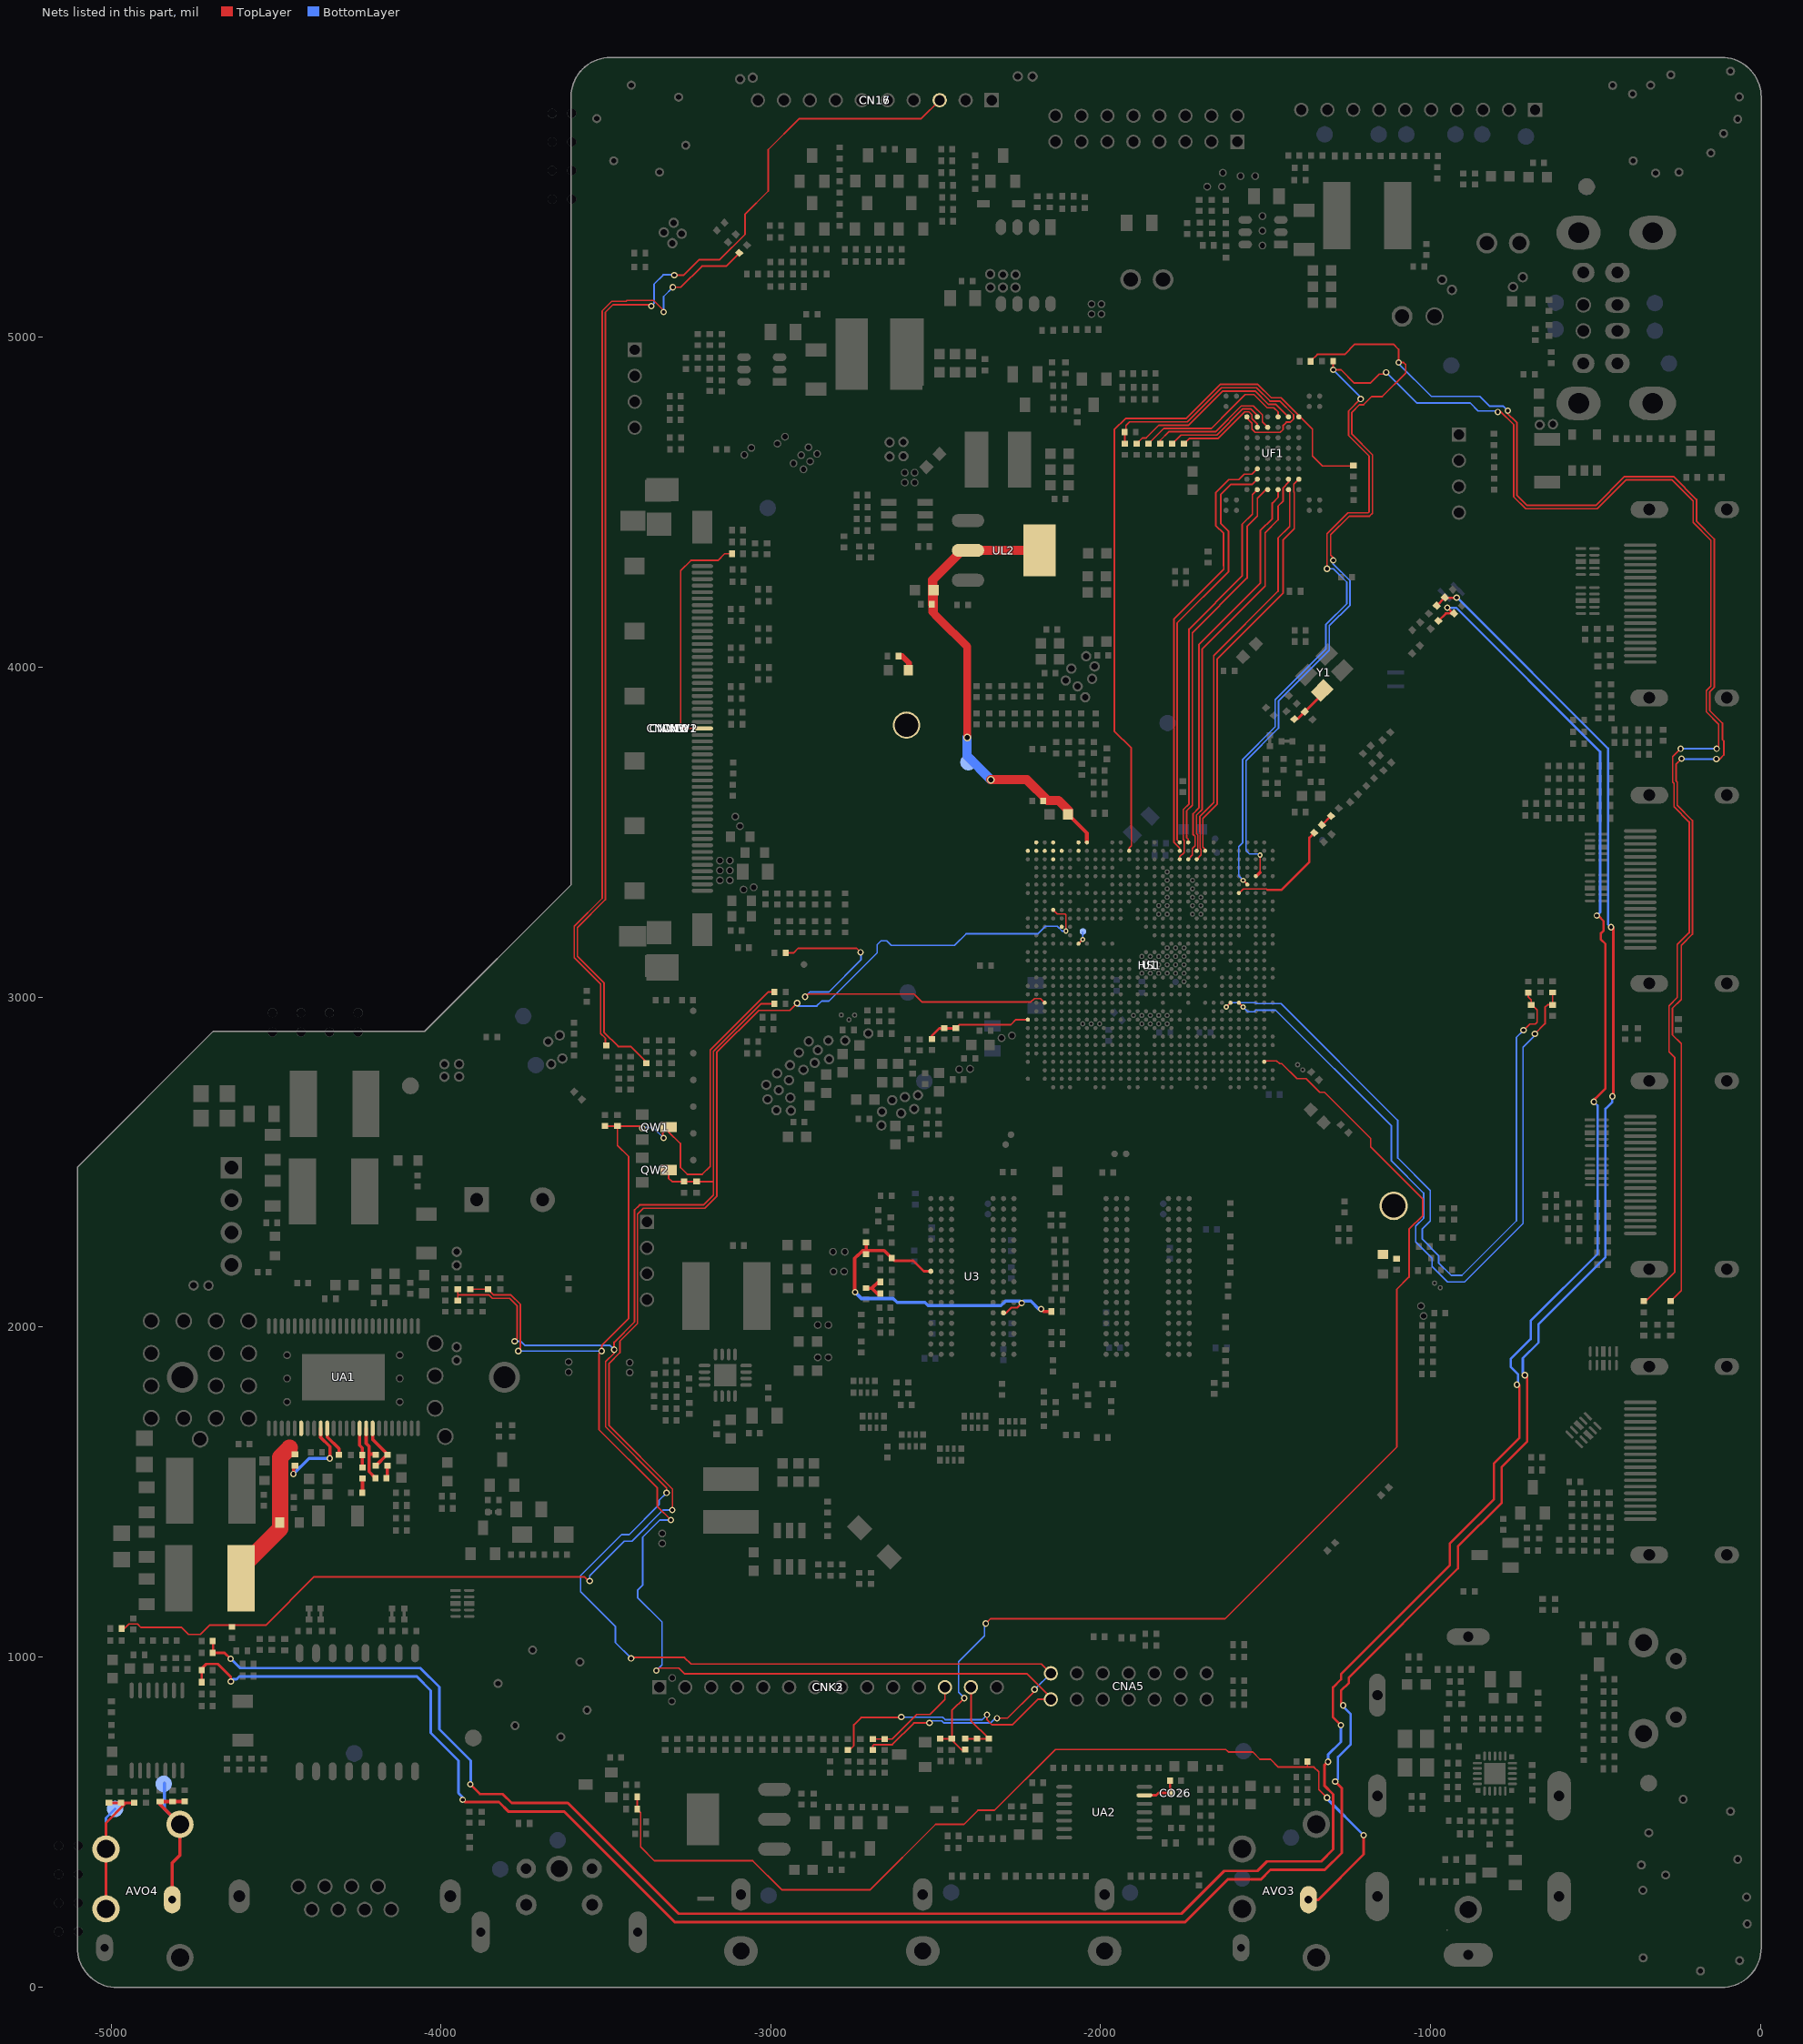
[diagram p0: the nets of this part, all layers, seen from the top]
# Altium PCB MISC86290.PcbDoc (part 24 of 31)
Units mil, origin at the board's own origin, x right, y up, seen from the top; angles counter-clockwise.
Board outline 5104.71 x 5851.49 mil, 2 copper layers (TopLayer, BottomLayer), stack 61.855 mil thick; 1026 components, 667 nets, 4280 pads, 2294 vias.

## Via types
v1: diameter 19.68, hole 11.81, TopLayer to BottomLayer, tented both sides, 1189 vias
v2: diameter 19.68/19.68 (per signal layer), hole 11.81, TopLayer to BottomLayer, tented both sides, 366 vias
v3: diameter 15.75, hole 7.87, TopLayer to BottomLayer, tented both sides, 348 vias
v4: diameter 23.62, hole 15.75, TopLayer to BottomLayer, tented both sides, 309 vias
v5: diameter 15.75/15.75 (per signal layer), hole 7.87, TopLayer to BottomLayer, tented both sides, 59 vias
v6: diameter 24/24 (per signal layer), hole 16, TopLayer to BottomLayer, tented both sides, 23 vias

## Nets (pads, with @x,y where several pads share a name; then routed paths per layer and width w, separated by ;. In a path a pad name is that pad's centre, name@x,y a point inside that pad or via, vN(x,y) a via of type N, cw(c..) or ccw(c..) an arc to the next point about the centre after c; other vN are vias at no path point) (continued)
LD_SPI_MISO: CN16.3 CN17.3 R126.2 | length 3844.1
  TopLayer w5: R126.2@-3380.73,2800.23 R126.2@-3377,2800.23 ; R126.2@-3380.73,2806.73 -3405.27,2831.27 -3405.41,2831.27 -3424.64,2850.5 -3462.64,2850.5 -3506,2893.86 -3506,3044 -3586.16,3124.16 -3586.16,3211.13 -3501.61,3295.68 -3501.61,5075.93 -3478.04,5099.5 -3367.03,5099.5 v1(-3362.28,5094.76) ; v1(-3292.5,5188.5) -3264.78,5188.5 -3217.28,5236 -3155,5236 -3078.09,5312.91 -3078.09,5373.62 -3008,5443.71 -3008,5569.22 -2914.37,5662.85 -2544.76,5662.85 CN16.3@-2488.15,5719.46
  BottomLayer w5: v1(-3362.28,5094.76) -3354,5103.04 -3354,5162.03 -3326.18,5189.84 -3293.84,5189.84 v1(-3292.5,5188.5)
LD_SPI_MOSI: R128.2 RG42.2 | length 2848.3
  TopLayer w5: R128.2@-3501.28,2854.6 -3501.28,2874.99 -3516,2889.72 -3516,3039.86 -3596.16,3120.02 -3596.16,3214.56 -3511.11,3299.61 -3511.11,5080.57 -3482.18,5109.5 -3438.5,5109.5 -3435.66,5112.34 -3355.34,5112.34 -3325,5082 v1(-3325,5077) ; v1(-3297,5152) -3272.99,5152 -3209,5216 -3136,5216 RG42.2@-3095.83,5256.17
  BottomLayer w5: v1(-3325,5077) -3325,5124 v1(-3297,5152)
LD_VSYNC: RG43.2 U1.L28 | length 1223.3
  TopLayer w3.94: -2211.22,2985.53 -2201.09,2995.67 -2182.4,2995.67 U1.L28@-2169.61,2982.87
  TopLayer w5: RG43.2@-2955.27,3134.5 -2930.5,3134.5 -2917,3148 -2740,3148 v1(-2728,3136) ; v1(-2896,3001) -2887.66,3009.34 -2566.38,3009.34 -2542.57,2985.53 ; -2541.32,2985.53 -2212.22,2985.53
  BottomLayer w5: v1(-2896,3001) -2881.34,3015.66 -2824.27,3015.66 -2726.88,3113.04 v1@-2726.88,3136
LED_G: CNK2.12 CNK3.12 RK37.1 RK40.2 | length 307.2
  TopLayer w5: RK40.2@-2691,750.73 RK37.1@-2655,750.73 -2631.91,750.73 -2557.14,825.5 -2517.53,825.5 -2471.98,871.05 CNK2.12@-2471.98,908 ; RK37.1@-2657.25,751 RK37.1@-2656.26,751.99
LED_OUT_IC: RK13.1 RK14.1 RK15.2 U1.D2 | length 3420.7
  TopLayer w3.94: U1.D2@-1502.05,2805.95 -1501.3,2806.69 -1466.58,2806.69 -1457.7,2797.81 -1450.53,2797.81
  TopLayer w5: RK15.2@-2487,751.73 RK13.1@-2451.5,751.73 RK13.1@-2451,751.73 ; RK14.1@-2415,718.27 -2421.27,718.27 -2451,748 RK13.1@-2451,751.73 ; v1(-2413.5,875) -2451,837.5 RK13.1@-2451,751.73 ; RK14.1@-2409.54,717.54 RK14.1@-2406,717.54 ; v1(-2348.5,1101) -2333.89,1115.61 -1623.03,1115.61 -1102.22,1636.41 -1102.22,2114.49 -1065.5,2151.22 -1065.5,2296.32 -1023.5,2338.32 -1023.5,2387.89 -1181.42,2545.82 -1181.42,2571.54 -1321.47,2711.58 -1336.14,2711.58 -1377.26,2752.7 -1405.42,2752.7 -1450.53,2797.81
  TopLayer w10: U1.D2@-1504.25,2803.74 -1503.46,2803.74 U1.D2@-1501.65,2805.55
  BottomLayer w5: v1(-2413.5,875) -2431,892.5 -2431,984.81 -2352,1063.82 -2352,1097.5 v1(-2348.5,1101)
LED_R: CK7.2 CNK2.13 CNK3.13 RK14.2 RK38.1 | length 250.2
  TopLayer w5: RK14.2@-2415,751.73 CK7.2@-2343,751.73 ; CNK2.13@-2393.24,908 -2393.24,806.47 CK7.2@-2339,752.23
LINEOUT_L: CO32.2 CO34.1 RO51.2 RO53.2 | length 8536.3
  TopLayer w7: v1(-1265,853) -1271.66,859.66 -1271.66,897.34 -1247.49,921.51 -1247.49,937.5 -917.09,1267.89 -917.09,1334.2 -784.28,1467.01 -784.28,1575.69 -706.88,1653.09 -706.88,1846.88 v1(-714,1854) ; RO51.2@-981.53,4186.64 -957.16,4211.01 v1(-920.84,4211.01) ; v1(-453,3212) -449,3212 -446,3209 -446,2699 v1(-449,2699)
  TopLayer w8: CO34.1@-4725.25,923.34 -4725.25,964.75 -4711.67,978.33 -4676.33,978.33 -4637.12,939.12 v1(-4637.12,925.06) ; v1(-3934.1,566.84) -3927.26,560 -3824.28,560 -3794.57,530.29 ; -3793.86,531 -3626.23,531 -3290.55,195.32 -1744.53,195.32 -1614.85,325 -1514.38,325 -1485.38,354 -1320.63,354 -1269,405.63 -1269,602 v1(-1289,622)
  BottomLayer w7: v1(-1289,622) -1280.66,630.34 -1280.66,696.34 -1241.66,735.34 -1241.66,825.66 -1265,849 v1(-1265,853) ; v1(-920.84,4211.01) -919.07,4211.01 -462,3753.94 -462,3221 v1(-453,3212) ; v1(-714,1854) -720.34,1860.34 -720.34,1905.34 -672.54,1953.13 -672.54,2008.81 -469.5,2211.85 -469.5,2661.44 -449,2681.94 v1(-449,2699)
  BottomLayer w8: v1(-4637.12,925.06) -4630.18,932 -4619.38,932 -4611.38,940 -4073.11,940 -4031,897.89 -4031,769.61 -3947,685.61 -3947,587 v1@-3934.1,574.1
LINEOUT_LL: AVO4.4 AVO4.5 DO32.K LINEOUT_L.1 RO38.2 RO40.2 | length 551.2
  TopLayer w8: AVO4.4@-5015.75,236.22 -5015.75,496.71 -4958.25,554.2 ; DO32.K@-5006.75,557.2 -5006.69,557.27 RO38.2@-4930.5,557.27
  BottomLayer w8: AVO4.5@-5015.75,417.32 -5015.75,511.25 LINEOUT_L.1@-4988,539
LINEOUT_MUTEN: RO44.1 RO45.2 U1.AB27 | length 4918.3
  TopLayer w3.9: U1.AB27@-2144.02,3264.37 -2131.22,3251.57 -2108,3251.57 -2105.63,3249.2 v3@-2105.63,3201.11
  TopLayer w5: RO44.1@-4968.43,1086 -4959.58,1086 -4945.95,1099.63 -4919.94,1099.63 -4909.32,1089 -4786.47,1089 -4765.32,1067.84 -4730,1067.84 -4701.84,1096 -4530.69,1096 -4384.19,1242.5 -3566,1242.5 v1@-3551.25,1227.75 ; v1(-3299,1445) -3298,1444 -3298,1508.55 -3490.34,1700.89 -3490.34,1889.66 -3457.5,1922.5 -3457.5,1957.07 -3404.25,2010.32 -3404.25,2342.24 -3386.49,2360 -3200,2360 -3163.91,2396.09 -3163.91,2832.55 -3036.46,2960 -2942.22,2960 v1(-2920.34,2981.88)
  BottomLayer w5: v1(-3549,1230) -3549,1245.7 -3444.05,1350.66 -3421.05,1350.66 -3326.71,1445 v1(-3299,1445) ; v1@-2916.8,2973 -2860.47,2973 -2845.47,2988 -2823.64,2988 -2677.5,3134.14 -2677.5,3159 -2666,3170.5 -2648.5,3170.5 -2635,3157 -2443.11,3157 -2408.1,3192.01 -2191.02,3192.01 -2167.92,3215.11 -2131.79,3215.11 -2117.08,3200.39 v3(-2105.63,3200.39)
LINEOUT_R: CO31.2 CO33.1 RO52.2 RO54.2 | length 8471.1
  TopLayer w7: v2(-1272,793) -1295.66,816.66 -1295.66,907.28 -1271.49,931.45 -1271.49,947.44 -941.09,1277.83 -941.09,1344.14 -808.28,1476.95 -808.28,1585.63 -730.88,1663.03 -730.88,1823.88 -732,1825 v1(-738,1825) ; RO52.2@-976.17,4140.83 -953.83,4163.17 RO54.2@-931.17,4163.17 ; v1(-949,4181) RO54.2@-931.17,4163.17 ; RO54.2@-928.83,4163.17 RO54.2@-931.17,4163.17 ; v1(-504.88,2682.46) -500,2677.58 -500,2692.97 -470,2722.97 -470,3161.06 -483.34,3174.4 -483.34,3194 -475,3202.34 -475,3230 -492,3247 v1(-496,3247)
  TopLayer w8: CO31.2@-4691.78,1048 CO31.2@-4690.78,1049 ; CO31.2@-4690.8,1048.84 -4690.8,1012.66 -4656.66,1012.66 v1(-4638,994) ; v1(-3910.84,613.58) -3882.26,585 ; -3881.8,585 -3882.26,585 ; v2(-1311,682) -1322,671 -1322,610 -1295,583 -1295,416.4 -1331.4,380 -1496.15,380 -1525.15,351 -1625.62,351 -1755.3,221.32 -3279.78,221.32 -3615.46,557 -3785.92,557 -3812.92,584 -3881.26,584 -3882.26,585
  BottomLayer w7: v1(-949,4181) -949.93,4180.07 -922.07,4180.07 -486,3744 -486,3257 v1(-496,3247) ; v1(-738,1825) -735,1828 -735,1857.06 -757.34,1879.4 -757.34,1902.28 -696.54,1963.07 -696.54,2018.75 -493.5,2221.79 -493.5,2671.08 v1(-504.88,2682.46)
  BottomLayer w8: v1(-4638,994) -4637,994 -4609,966 -4062.34,966 -4005,908.66 -4005,780.38 -3910,685.38 -3910,614.42 v1(-3910.84,613.58) ; v2(-1311,682) -1311,703 -1272,742 v2(-1272,793)
LINEOUT_RR: AVO4.3 AVO4.6 DO31.K LINEOUT_R.1 RO37.2 RO39.2 | length 557.7
  TopLayer w10: AVO4.6@-4814.96,263.78 -4814.96,375.04 -4791.34,398.66 AVO4.3@-4791.34,492.13 -4851.5,552.29 DO31.K@-4851.5,561.27 RO39.2@-4813.5,561.27 RO37.2@-4781.73,561.27 ; AVO4.3@-4803,503 AVO4.3@-4795.02,495.02
  BottomLayer w10: LINEOUT_R.1@-4838.5,617 -4838.5,539.29 AVO4.3@-4791.34,492.13
LINN: CO26.2 RO56.2 UA2.13 | length 111.1
  TopLayer w8: UA2.13@-1867.44,580.18 -1831.32,580.18 -1824.5,587 CO26.2@-1789.73,587 ; CO26.2@-1789.73,593.89 RO56.2@-1789.73,624.5
LOCKN_TX: CNW1.26 CNW2.26 CNW3.26 CNW12.26 RW10.1 | length 714.4
  TopLayer w5: CNW3.26@-3207.67,3814.53 -3261.78,3814.53 -3273.5,3826.25 -3273.5,4292.75 -3242.26,4324 -3160.25,4324 -3140.25,4344 RW10.1@-3117.52,4344
LOG_RX: R72.2 RH38.2 U1.AE4 | length 6107.2
  TopLayer w5: v3(-1568.23,3353.94) U1.AE4@-1555.43,3341.14 ; v1(-1313.94,4298.79) -1313.94,4404.84 -1250.78,4468 -1189.5,4468 -1186,4471.5 -1186,4640 -1248.5,4702.5 -1248.5,4777.05 -1211.77,4813.77 v1(-1211.77,4813.28) ; R72.2@-1295.27,4929.27 R72.2@-1295.27,4928 -1295.27,4902.27 -1271.97,4902.27 -1231.33,4861.63 -1183.33,4861.63 -1155.96,4889 -1139.63,4889 v1(-1134.68,4893.95) ; v1@-796,4777 -789.72,4777 -748,4735.28 -748,4517 -711.7,4480.7 -494.96,4480.7 -407.66,4568 -267.34,4568 -204,4504.66 -204,4438.75 -150,4384.75 -150,3943.14 -164,3929.14 -164,3865 -126.66,3827.66 -126.66,3758.84 v1(-132.5,3753) ; RH38.2@-353.77,2072.23 -259.66,2166.34 -259.66,2816.66 -277,2834 -277,2974 -252,2999 -252,3159.14 -216,3195.14 -216,3530.96 -262,3576.96 -262,3648.14 -266,3652.14 -266,3729 v1(-242,3753)
  BottomLayer w3.94: -1579.62,3458 -1582.01,3455.62 -1582.01,3367.72 v3(-1568.23,3353.94)
  BottomLayer w5: -1579.62,3458 -1569.5,3468.13 -1569.5,3721.06 -1471,3819.56 -1471,3901.64 -1317,4055.64 -1317,4130 -1254,4193 -1254,4258 -1294.79,4298.79 v1(-1313.94,4298.79) ; v1(-1295,4902) -1295,4901.26 -1211.77,4818.03 v1(-1211.77,4813.28) ; v1(-1134.68,4893.95) -1042.24,4801.5 -880.21,4801.5 -855.71,4777 v1@-796,4777 ; v1(-242,3753) v1@-134.5,3753
  other v1: -796,4774
LOG_TX: R73.2 RH37.2 U1.AF3 | length 6263
  TopLayer w3.94: -1517.05,3378.06 v3@-1517.05,3427.11
  TopLayer w5: R73.2@-1363.27,4927.5 -1363.27,4928.42 -1343.19,4948.5 -1260.32,4948.5 -1229.32,4979.5 -1112.5,4979.5 -1097,4964 v1(-1097,4924) -1082,4924 -1075.34,4917.34 -1075.34,4891.84 -1146.56,4820.63 -1178.37,4820.63 -1203.06,4795.94 -1215.46,4795.94 -1238.5,4772.9 -1238.5,4706.64 -1176,4644.14 -1176,4467.36 -1185.36,4458 -1246.64,4458 -1303,4401.64 -1303,4340 -1295,4332 v1(-1295,4324) ; v1@-770.5,4773.5 -738,4741 -738,4521.14 -707.56,4490.7 -499.1,4490.7 -411.8,4578 -263.2,4578 -194,4508.8 -194,4442.89 -140,4388.89 -140,3939 -154,3925 -154,3869.14 -115.32,3830.46 -115.32,3781 -111,3776.68 -111,3734 -123,3722 v1(-133.5,3722) v1@-134.5,3722 ; RH37.2@-272,2078.23 -239.66,2110.57 -239.66,2858.66 -267,2886 -267,2966 -239.66,2993.34 -239.66,3157.34 -206,3191 -206,3535.11 -252,3581.11 -252,3652.28 -256,3656.28 -256,3706 v1(-239,3723)
  TopLayer w10: U1.AF3@-1529.84,3366.73 -1528.38,3366.73 -1517.05,3378.06
  BottomLayer w5: v3@-1516.85,3434.11 -1549,3434.11 -1559.5,3444.61 -1559.5,3716.92 -1461,3815.42 -1461,3897.5 -1307,4051.5 -1307,4125.86 -1244,4188.86 -1244,4262.14 -1296,4314.14 -1296,4323 v1(-1295,4324) ; v1@-1097,4921 -997.5,4821.5 -851.16,4821.5 -821.66,4792 -780,4792 v1(-766,4778) ; v1@-238,3722 v1(-133.5,3722)
  other v3: -1517.05,3430.71
MCP_TEST: MCP_TEST.1 U1.V24 | length 41.8
  TopLayer w3.94: U1.V24@-2067.24,3162.01 v3(-2054.45,3174.8)
  BottomLayer w3.94: v3@-2054,3175.25 MCP_TEST.1@-2054,3199
MI2C_SCL: CNA5.13 D5.K QW2.D R122.1 R200.1 RA14.1 RK40.1 RW395.2 | length 5344.8
  TopLayer w5: RA14.1@-3949,2079.73 R122.1@-3949,2114.27 ; -3948.67,2097.67 -3854.86,2097.67 -3844.22,2087.03 -3792.03,2087.03 -3769.34,2064.34 -3769.34,1964.23 ; v1@-3423.66,998.16 -3261.93,998.16 -3242.08,978.31 -2179.53,978.31 CNA5.13@-2151.22,950 ; v1(-3316,1497) -3316,1512.41 -3501,1697.41 -3501,1894.86 -3475,1920.86 v1(-3475,1931) -3475,1953.71 -3413.25,2015.46 -3413.25,2354.75 -3398,2370 -3204.14,2370 -3173.91,2400.24 -3173.91,2835.99 -3159.26,2850.63 ; QW2.D@-3310,2476 -3310,2451 -3299.73,2440.73 RW395.2@-3263,2440.73 -3176.17,2440.73 ; -3170.5,2839.39 -3159.26,2850.63 ; R200.1@-2988.96,2979.5 -3030.39,2979.5 -3159.26,2850.63 ; RK40.1@-2691,717.27 -2691,730.5 -2687.5,734 -2631.84,734 -2566.34,799.5 v1(-2519,799.5) v1@-2517.98,798.48 ; v1(-2314.5,814) -2282.53,814 v1@-2198.01,898.51
  BottomLayer w5: v1(-3776.68,1956.88) -3758.54,1956.88 -3746.5,1944.84 ; -3746.5,1944.34 -3488.34,1944.34 v1(-3475,1931) ; v1(-3423.66,995.11) -3423.66,995.84 -3471.59,1043.78 -3471.59,1092.25 -3576.5,1197.16 -3576.5,1246.49 -3452.33,1370.66 -3429.34,1370.66 -3339,1460.99 -3339,1474 v1(-3316,1497) ; v1@-2512.66,805.84 -2481.82,805.84 -2475.47,799.5 -2334,799.5 v1@-2319.5,814 ; v1@-2200.22,901 CNA5.13@-2151.22,950
  other v1: -2200.5,901
MI2C_SDA: CNA5.14 D4.K QW1.D R124.1 R201.1 RA12.1 RK41.1 RW393.2 | length 5531
  TopLayer w5: R124.1@-3911,2114.27 RA12.1@-3857.35,2114.29 ; RA12.1@-3857.35,2114.29 -3840.08,2097.03 -3787.88,2097.03 -3759.34,2068.48 v1@-3759.34,1933.16 ; RW393.2@-3503,2609.27 D4.K@-3465,2609.27 ; -3432.25,2024.75 -3513,1944 v1(-3513,1927) -3521,1919 -3521,1689.12 -3344,1512.12 -3344,1456 v1(-3303,1415) ; -3431.25,2025.75 -3431.25,2517.04 -3465,2550.79 D4.K@-3465,2609.27 ; v1(-3389.5,2602.5) -3396.27,2609.27 D4.K@-3465,2609.27 ; -3339.5,966 -3279,966 -3261.32,948.31 -2222.98,948.31 CNA5.14@-2151.22,876.55 ; v1(-3325,2573) -3327.5,2575.5 -3327.5,2588.5 QW1.D@-3310,2606 -3310,2592.14 -3274,2556.14 -3274,2483.72 -3253.28,2463 -3207.86,2463 -3183.91,2486.95 -3183.91,2839.42 -3007.33,3016 R201.1@-2988.73,3016 ; RK41.1@-2766.5,717.77 -2761.58,717.77 -2748.5,730.85 -2748.5,794.01 -2726.51,816 v1@-2604.5,816 ; v1(-2344.5,824.14) -2344.5,809 -2329.5,794 -2268,794 -2190.74,871.26 CNA5.14@-2151.22,871.26
  BottomLayer w5: v1(-3765.5,1927) v1(-3513,1927) ; v1(-3389.5,2602.5) -3387.66,2604.34 -3356.34,2604.34 v1(-3325,2573) ; v1(-3347,958.5) -3329.72,975.78 -3329.72,1105.93 -3404,1180.22 -3404,1202 -3388.75,1217.25 -3388.75,1362.39 -3336.14,1415 v1(-3303,1415) ; v1@-2603.84,816.84 -2478.67,816.84 -2471.33,809.5 -2359.14,809.5 v1(-2344.5,824.14)
  other v1: -2604.5,817.5
MIC_OFF_BTNN: U1.Y26
MOD_1V2: C25.2 C26.1 CL13.2 CL25.2 MOD_1V2.1 U1.AK23 UL2.2 UL2.4 | length 1528.1
  TopLayer w12: C25.2@-2098.01,3553.26 -2041.65,3496.91 U1.AK23@-2041.65,3469.09
  TopLayer w24: -2511.03,4213.23 -2511.03,4168.53 -2506,4163.5 ; CL13.2@-2507.19,4234 -2506,4232.81 -2506,4163.5 ; -2502.25,4159.75 -2489.75,4147.25 ; v4(-2405,3787) -2405,4062.5 -2489.75,4147.25 ; -2506,4163.5 -2489.75,4147.25
  TopLayer w28: CL25.2@-2509.25,4191 -2509.25,4264.77 -2419.59,4354.43 UL2.2@-2402.27,4354.43 UL2.4@-2202.73,4354.43 ; v4(-2333,3659.11) -2224,3659.11 -2161.39,3596.5 -2128,3596.5 -2098.01,3566.51 C25.2@-2098.01,3553.26
  BottomLayer w28: v4(-2405,3787) -2405,3731.11 v4(-2333,3659.11)
MOD_TX_N08: U1.AJ29
MOD_TX_N09: U1.AJ28
MOD_TX_N10: U1.AJ27
MOD_TX_N11: U1.AJ26
MOD_TX_N13: U1.AK24
MOD_TX_P08: U1.AJ30
MOD_TX_P09: U1.AK29
MOD_TX_P10: U1.AK27
MOD_TX_P11: U1.AH27
MOD_TX_P13: U1.AJ24
MSTV_SCL: D41.K R140.2 U1.L5 | length 2227.5
  TopLayer w3.94: U1.L5@-1581.02,2982.87 v3(-1568.23,2970.08)
  TopLayer w5: v1@-683.59,2888.72 -653,2919.31 -653,2969 -645.27,2976.73 D41.K@-630,2976.73 R140.2@-630,3014.27
  BottomLayer w3.94: v3(-1568.23,2970.08) -1554.45,2956.3 -1533.86,2956.3 -1529.62,2960.53 -1524.41,2960.53
  BottomLayer w5: -1524.41,2960.53 -1469.89,2960.53 -1118.51,2609.16 -1118.51,2503.31 -1021,2405.8 -1021,2330 -1044.99,2306.01 -1044.99,2257.66 -995.66,2208.33 -995.66,2183.9 -948.41,2136.66 -896.85,2136.66 -719.68,2313.82 -719.68,2847.86 v1@-683.63,2883.92
  other v1: -683.63,2888.72
MSTV_SDA: D40.K R141.2 U1.L6 | length 2256.1
  TopLayer w3.94: v3(-1619.41,2970.08) U1.L6@-1606.61,2982.87
  TopLayer w5: v1(-718.32,2899.62) -699.38,2918.55 -682.04,2918.55 -676.67,2923.92 -676.67,2961.67 -691.73,2976.73 D40.K@-695,2976.73 -695,2992 -704,3001 R141.2@-704,3013.77
  BottomLayer w3.94: v3(-1619.41,2970.08) -1605.63,2983.86 -1530.55,2983.86 -1527.22,2980.53
  BottomLayer w5: -1527.22,2980.53 -1453.53,2980.53 -1099.61,2626.61 -1099.61,2512.7 -1001,2414.08 -1001,2321.72 -1024.99,2297.73 -1024.99,2265.94 -975.66,2216.61 -975.66,2194.74 -937.58,2156.66 -905.13,2156.66 -739.68,2322.11 -739.68,2878.25 v1(-718.32,2899.62)
NAND_AD0: U1.AJ12 UF1.H4 | length 1319.8
  TopLayer w3.94: -1776.89,3468.11 -1760.16,3451.38 U1.AJ12@-1760.16,3443.5
  TopLayer w4.92: -1778.22,3469.44 -1778.22,4145.78 -1627.25,4296.75 -1627.25,4308
  TopLayer w5: -1627.25,4308 -1627.25,4405.87 -1651.27,4429.89 -1651.27,4529.09 -1611.25,4569.11 -1581.25,4569.11 -1564.83,4585.52 -1541.36,4585.52 UF1.H4@-1525.24,4601.65
NAND_AD1: U1.AK12 UF1.J4 | length 1262.9
  TopLayer w5: U1.AK12@-1760.16,3469.09 -1768.22,3477.16 -1768.22,4134.78 -1612.23,4290.77 -1612.23,4412.09 -1636.25,4436.11 -1636.25,4523.87 -1605.86,4554.26 -1541.13,4554.26 UF1.J4@-1525.24,4570.15
NAND_AD2: U1.AH12 UF1.K4 | length 1220
  TopLayer w3.94: U1.AH12@-1760.16,3417.91 -1760.16,3425.79 -1747.36,3438.58 -1747.36,3475.67 -1749.72,3478.03 -1749.72,3487.2
  TopLayer w5: -1749.72,3487.2 -1749.72,3568.55 -1732.22,3586.05 -1732.22,4115.78 -1571.25,4276.75 -1571.25,4433.11 -1539.89,4464.47 -1539.89,4524 UF1.K4@-1525.24,4538.65
NAND_AD3: U1.AK11 UF1.K5 | length 1176.5
  TopLayer w5: U1.AK11@-1734.57,3469.09 -1734.57,3477.87 -1739.72,3483.03 -1739.72,3564.39 -1722.22,3581.89 -1722.22,4104.78 -1556.25,4270.75 -1556.25,4427.11 -1524.87,4458.48 -1524.87,4512.48 -1498.71,4538.65 UF1.K5@-1493.75,4538.65
NAND_AD4: U1.AH11 UF1.K6 | length 1238.4
  TopLayer w3.94: U1.AH11@-1733.58,3418.9 -1721.77,3430.71 -1721.77,3450.39 -1713.9,3458.27 -1713.9,3487.2 -1717.69,3491
  TopLayer w5: U1.AH11@-1734.57,3417.91 U1.AH11@-1733.58,3418.9 ; -1717.69,3491 -1719.72,3493.03 -1719.72,3556.07 -1702.22,3573.57 -1702.22,4068.78 -1516.25,4254.75 -1516.25,4414.11 -1479.77,4450.59 -1479.77,4497.59 -1462.25,4515.11 UF1.K6@-1462.25,4538.65
NAND_AD5: U1.AJ10 UF1.J7 | length 1246.7
  TopLayer w3.94: U1.AJ10@-1708.98,3443.5 -1706.02,3443.5 -1706.02,3491.83 -1708.36,3494.17
  TopLayer w5: -1708.36,3494.17 -1709.72,3495.53 -1709.72,3551.91 -1692.22,3569.41 -1692.22,4055.78 -1501.25,4246.75 -1501.25,4408.11 -1462.27,4447.09 -1462.27,4489.09 -1446.87,4504.48 -1446.87,4544.28 -1430.76,4560.39 UF1.J7@-1430.76,4570.15
NAND_AD6: U1.AH10 UF1.K7 | length 1241.8
  TopLayer w3.94: U1.AH10@-1708.98,3417.91 -1696.18,3430.71 -1696.18,3448.43 -1698.15,3450.39 -1698.15,3498.96 -1699.72,3500.53
  TopLayer w4.92: -1699.72,3500.53 -1699.72,3547.24 -1657.22,3589.74 -1657.22,3977.29
  TopLayer w5: -1657.22,3977.29 -1657.22,4035.78 -1462.25,4230.75 -1462.25,4392.11 -1427.27,4427.09 -1427.27,4535.16 UF1.K7@-1430.76,4538.65
NAND_AD7: U1.AJ9 UF1.J8 | length 1251
  TopLayer w3.94: U1.AJ9@-1683.39,3443.5 -1683.39,3447.44 -1690.28,3454.33 -1690.28,3541.75 -1675.33,3556.69
  TopLayer w5: -1675.33,3556.69 -1647.22,3584.8 -1647.22,4024.78 -1447.25,4224.75 -1447.25,4386.11 -1413.49,4419.86 -1413.49,4530.97 -1414.63,4532.11 -1414.63,4554.78 UF1.J8@-1399.26,4570.15
NAND_ALE: RF3.2 UF1.C4 | length 314.6
  TopLayer w5: RF3.2@-1783.25,4677.57 -1756.82,4704 -1648.22,4704 -1568.71,4783.5 -1545.23,4783.5 -1525.24,4763.51 UF1.C4@-1525.24,4759.13
NAND_CEZ: RF7.2 UF1.C6 | length 492.1
  TopLayer w5: RF7.2@-1855.25,4677.57 -1808.82,4724 -1664.61,4724 -1604.35,4784.25 -1572.86,4815.75 -1572.86,4816.14 -1562,4827 -1535.28,4827 -1495.28,4787 -1475,4787 -1462.25,4774.25 UF1.C6@-1462.25,4759.13
NAND_CLE: RF4.2 UF1.D5 | length 418.9
  TopLayer w5: RF4.2@-1819.25,4677.57 -1819.25,4688.11 -1793.36,4714 -1652.36,4714 -1573.85,4792.5 -1536.87,4792.5 -1509.76,4765.39 -1509.76,4743.64 UF1.D5@-1493.75,4727.63
NAND_RBZ: RF2.1 U1.AJ18 UF1.C8 | length 2235.5
  TopLayer w3.94: U1.AJ18@-1913.7,3443.5 -1913.7,3451.38 -1906.81,3458.27 -1906.81,3511 -1907.22,3511.42
  TopLayer w4.92: -1907.22,3511.42 -1907.22,3722
  TopLayer w5: -1907.22,3722 -1907.22,3755.22 -1958.95,3806.95 -1958.95,4720.05 -1925,4754 -1741.72,4754 -1638.22,4857.49 -1523.35,4857.49 -1482.85,4817 -1452.74,4817 -1399.26,4763.51 UF1.C8@-1399.26,4759.13 ; UF1.C8@-1397.26,4761.13 -1358.25,4722.11 -1358.25,4640.25 -1328.25,4610.25 RF2.1@-1233.16,4610.25
NAND_REZ: RF6.2 UF1.D4 | length 283.7
  TopLayer w5: RF6.2@-1739.71,4685.11 -1730.82,4694 -1644.07,4694 -1563.57,4774.5 -1550.37,4774.5 -1541.36,4765.5 -1541.36,4761.15 -1541.32,4761.11 -1541.25,4761.11 -1541.25,4753.4 -1525.24,4737.39 UF1.D4@-1525.24,4727.63
NAND_WEZ: RF5.2 UF1.C7 | length 559.2
  TopLayer w5: RF5.2@-1891.25,4677.57 -1873.71,4695.11 -1862.25,4695.11 -1823.36,4734 -1733.43,4734 -1629.94,4837.49 -1531.63,4837.49 -1491.14,4797 -1468.63,4797 UF1.C7@-1430.76,4759.13
NAND_WPZ: RF1.2 RF8.2 UF1.C3 | length 856.4
  TopLayer w5: RF8.2@-1927.25,4677.57 RF1.2@-1927.25,4713.11 -1923.25,4717.11 -1923.25,4733.11 -1912.36,4744 -1737.58,4744 -1634.08,4847.49 -1527.49,4847.49 -1487,4807 -1456.89,4807 -1415.38,4765.5 -1415.38,4752.76 -1425.14,4743 -1437.13,4743 -1446.87,4733.26 -1446.87,4721.26 -1455.88,4712.26 -1531.61,4712.26 -1541.36,4722.01 -1541.36,4739.37 -1556.74,4754.75 UF1.C3@-1556.74,4759.13
NetAVO3_6: AVO3.6 RO26.2 RO27.2 RO28.1 | length 3023.1
  TopLayer w5: RO27.2@-3405.05,575.53 RO28.1@-3405.05,538.53 -3394.5,527.98 -3394.5,423.5 -3353,382 -3055,382 -2967,294 -2698.73,294 -2500.39,492.34 -2414.66,492.34 -2372,535 -2322,535 -2137.68,719.32 -1620.82,719.32 -1613.25,711.75 -1539.5,711.75 -1517.25,689.5 -1485.45,689.5 -1461.65,665.7 -1374,665.7 ; -1374,666.43 -1374,665.7 ; -1373.27,666.43 RO26.2@-1373.27,682.5 ; v1(-1314,573) -1339,598 -1339,651.26 -1353.44,665.7 -1374,665.7
  TopLayer w8: AVO3.6@-1370.08,263.78 -1340.14,263.78 -1203,400.92 v1(-1203,459) ; v1(-1314,573) v1@-1314,578.81
  BottomLayer w8: v1(-1314,573) -1314,570 v1(-1203,459)
NetC55_1: C55.1 R39.2 | length 38.7
  TopLayer w7: C55.1@-1329.17,3521.83 R39.2@-1301.83,3549.17
NetC55_2: C55.2 U1.AD5 | length 342.1
  TopLayer w3.94: U1.AD5@-1578,3318.11 -1567.91,3328.2 -1495.97,3328.2
  TopLayer w7: -1494.08,3325.75 -1451.52,3325.75 -1367.5,3409.77 -1367.5,3483.5 C55.2@-1352.83,3498.17
NetC57_1: C57.1 R208.2 Y1.1 | length 115.1
  TopLayer w8: R208.2@-1413.15,3842.85 -1403.81,3842.85 C57.1@-1381.3,3865.36 Y1.1@-1329.01,3917.65
NetC59_2: C59.2 R46.1 R47.2 U1.J30 | length 320
  TopLayer w5: C59.2@-2439.01,2906.13 -2429.11,2916.03 -2272.95,2916.03 -2257.29,2931.69 U1.J30@-2220.79,2931.69
  TopLayer w8: R46.1@-2511.84,2873.05 -2511.84,2883.4 -2489.61,2905.63 R47.2@-2474.76,2905.63 ; R47.2@-2473.51,2905.63 C59.2@-2439.01,2905.63
NetC100_2: C100.2 C101.2 R103.1 R104.2 U3.H1 U3.M8 | length 1143.7
  TopLayer w5.91: U3.M8@-2294.61,2042.91 -2286.73,2042.91 -2270.98,2058.66 -2253.27,2058.66 v2(-2239.49,2072.44)
  TopLayer w7.87: C101.2@-2634.12,2208.55 -2626.12,2200.55 -2568.24,2200.55 -2536.59,2168.9 U3.H1@-2515.08,2168.9
  TopLayer w9.84: v2@-2745.97,2105.53 -2745.97,2208.58 -2721.75,2231.52 -2721.37,2231.89 -2720.12,2231.89 ; -2744.72,2208.58 -2721.16,2230.9 -2720.12,2231.89 ; R104.2@-2711.21,2220.39 -2710.97,2220.63 -2710.97,2231.89 ; R103.1@-2711.21,2257.16 -2710.97,2256.93 -2710.97,2231.89 ; -2657.74,2231.89 -2710.97,2231.89 ; -2656.5,2231.89 -2633.64,2209.03 C101.2@-2632.87,2208.27 ; v2(-2180.43,2054.72) -2172.56,2046.85 C100.2@-2149.25,2046.85 ; -2720.12,2231.89 -2710.97,2231.89
  BottomLayer w9.84: v2(-2744.72,2105.53) -2725.41,2086.22 -2629.25,2086.22 -2617.44,2074.41 -2532.8,2074.41 -2522.95,2064.57 -2302.48,2064.57 -2288.7,2078.35 -2245.39,2078.35 v2(-2239.49,2072.44) -2233.58,2078.35 -2211.93,2078.35 -2188.31,2054.72 v2(-2180.43,2054.72)
NetC102_2: C102.2 R105.1 R106.1 | length 74.9
  TopLayer w9.84: C102.2@-2711.21,2118.03 -2710.89,2117.72 -2693.49,2117.72 ; R105.1@-2674.12,2100.98 -2674.12,2098.35 -2693.49,2117.72 ; R106.1@-2674.12,2136.42 -2693.49,2118.03 -2693.49,2117.72
NetC164_1: C164.1 UA1.10 | length 93
  TopLayer w10: UA1.10@-4344.96,1692.73 -4344.96,1666.75 -4309.18,1630.96 C164.1@-4309.18,1614.6
NetC200_1: C200.1 C202.2 HS1.1 | length 47.1
  TopLayer w17: C202.2@-2610.32,4034 -2602,4034 -2581,4013 C200.1@-2581,4003.88
NetC201_2: C201.2 C205.2 HS1.2
NetCA3_1: CA3.1 RA6.1 UA1.16 | length 181.6
  TopLayer w10: UA1.16@-4226.85,1692.73 -4226.85,1647.1 -4217.91,1638.16 -4217.91,1614.6 ; CA3.1@-4198.96,1614.6 -4217.91,1614.6 ; RA6.1@-4198.48,1541.81 -4217.91,1561.23 -4217.91,1614.6
NetCA3_2: CA3.2 CA5.2 UA1.17 | length 148.8
  TopLayer w10: UA1.17@-4207.17,1692.73 -4207.17,1658.81 CA5.2@-4162.96,1614.6 ; CA3.2@-4198.96,1581.13 CA3.2@-4196.42,1581.13 ; CA3.2@-4197.75,1579.08 -4164.29,1612.54 CA5.2@-4161.75,1612.54
NetCA5_1: CA5.1 RA6.2 | length 37.8
  TopLayer w10: RA6.2@-4164.23,1543.87 -4162.96,1545.13 CA5.1@-4162.96,1581.13
NetCA7_2: CA7.2 CA11.2 UA1.15 | length 118.4
  TopLayer w10: UA1.15@-4246.54,1692.73 -4246.54,1641.72 -4238.45,1633.63 -4238.45,1578.37 CA11.2@-4238.95,1577.87
NetCA11_1: CA11.1 RA8.2 | length 43.8
  TopLayer w12: RA8.2@-4239.02,1497.81 -4237.75,1499.08 CA11.1@-4237.75,1541.08
NetCA13_1: CA13.1 UA1.9 | length 263.1
  TopLayer w10: v1(-4447.25,1554.31) -4447.25,1575.58 CA13.1@-4442.75,1580.08 CA13.1@-4440.02,1580.08 ; UA1.9@-4364.65,1692.73 -4364.65,1665.22 -4336.83,1637.4 v1(-4336.85,1601.41)
  BottomLayer w10: v1(-4447.25,1554.31) -4400.15,1601.41 v1(-4336.85,1601.41)
NetCA13_2: CA13.2 LA1.1 RA16.1 UA1.6 | length 464.3
  TopLayer w40: -4463.79,1634.58 -4461.9,1636.46
  TopLayer w50: LA1.1@-4606.25,1233 LA1.1@-4606.25,1238 -4606.25,1269.75 -4487.39,1388.61 -4487.39,1605.32 -4459.08,1633.64